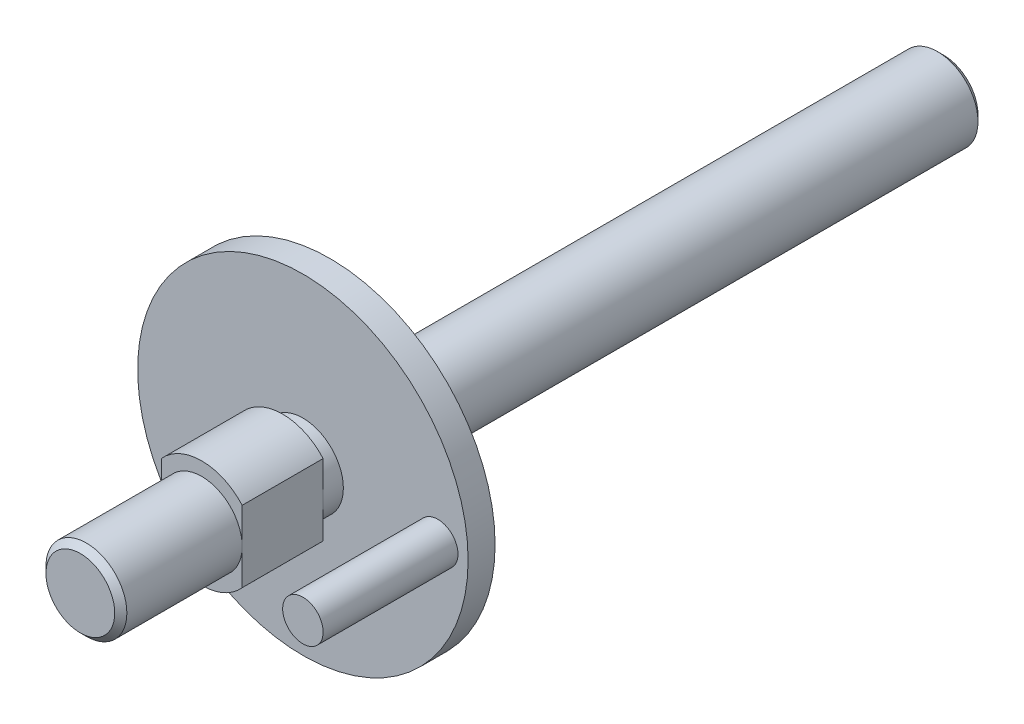
from build123d import *

# Parameters (mm, degrees)
SKETCH1_R           = 6
BOSS_EXTRUDE1_DEPTH = 91
SKETCH2_R           = 24.5
BOSS_EXTRUDE2_DEPTH = 4
SKETCH3_R           = 6
BOSS_EXTRUDE3_DEPTH = 3
BOSS_EXTRUDE4_DEPTH = 12
SKETCH5_R           = 6
BOSS_EXTRUDE5_DEPTH = 18
CHAMFER1_SIZE       = 0.9
SKETCH6_R           = 3
BOSS_EXTRUDE6_DEPTH = 20


with BuildPart() as part:
    # Sketch1 → Boss-Extrude1 (new body)
    with BuildSketch(Plane.XY):
        Circle(SKETCH1_R)
    extrude(amount=BOSS_EXTRUDE1_DEPTH)

    # Sketch2 → Boss-Extrude2 (add)
    with BuildSketch(Plane.XY.offset(91)):
        Circle(SKETCH2_R)
    extrude(amount=BOSS_EXTRUDE2_DEPTH)

    # Sketch3 → Boss-Extrude3 (add)
    with BuildSketch(Plane.XY.offset(95)):
        Circle(SKETCH3_R)
    extrude(amount=BOSS_EXTRUDE3_DEPTH)

    # Sketch4 → Boss-Extrude4 (add)
    with BuildSketch(Plane.XY.offset(98)):
        with BuildLine():
            Line((6, 5.291502622), (6, -5.291502622))
            ThreePointArc((6, -5.291502622), (0, -8), (-6, -5.291502622))
            Line((-6, -5.291502622), (-6, 5.291502622))
            ThreePointArc((-6, 5.291502622), (0, 8), (6, 5.291502622))
        make_face()
    extrude(amount=BOSS_EXTRUDE4_DEPTH)

    # Sketch5 → Boss-Extrude5 (add)
    with BuildSketch(Plane.XY.offset(110)):
        Circle(SKETCH5_R)
    extrude(amount=BOSS_EXTRUDE5_DEPTH)

    # Chamfer1
    chamfer1_edges = [part.edges().sort_by_distance(p)[0] for p in [
        (-6, 0, 0),
        (-6, 0, 128),
    ]]
    chamfer(chamfer1_edges, length=CHAMFER1_SIZE)

    # Sketch6 → Boss-Extrude6 (add)
    with BuildSketch(Plane.XY.offset(95)):
        with Locations((20, 0)):
            Circle(SKETCH6_R)
    extrude(amount=BOSS_EXTRUDE6_DEPTH)


solid = part.part
